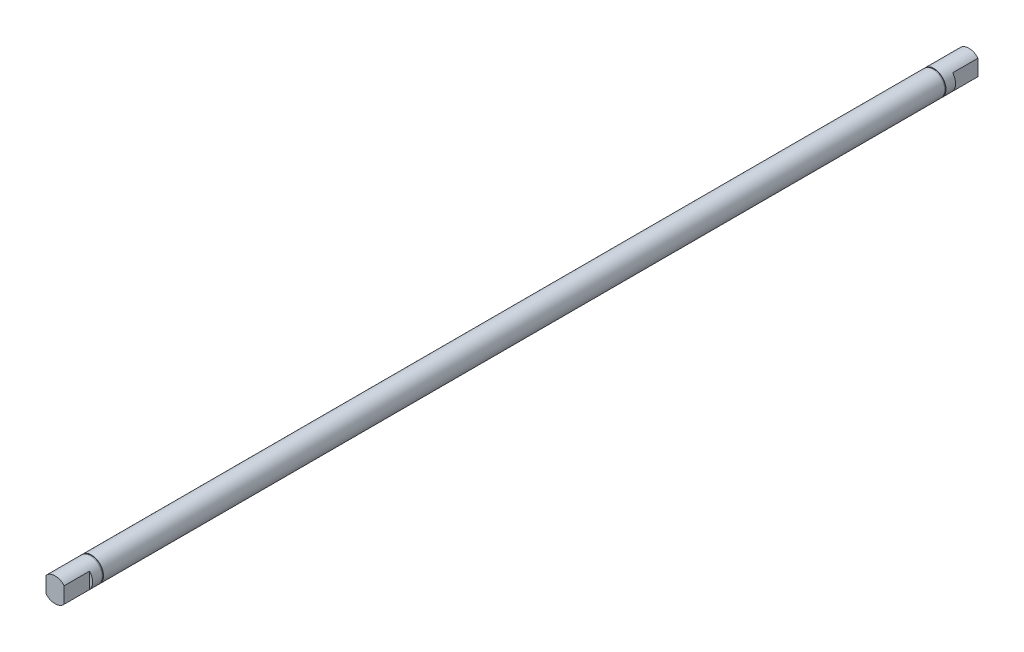
from build123d import *

# Parameters (mm, degrees)
SKETCH_1_R          = 10
EXTRUDE_1_DEPTH     = 377.5
SKETCH_2_W          = 20.903935991
SKETCH_2_H          = 21
CUT_EXTRUDE_1_DEPTH = 25
CUT_EXTRUDE_START   = -30
SKETCH_5_R          = 10
SKETCH_5_R_2        = 9.5
CUT_EXTRUDE_2_DEPTH = 1.1


with BuildPart() as part:
    # 草图1 → 凸台-拉伸1 (new, symmetric)
    with BuildSketch(Plane.XY):
        Circle(SKETCH_1_R)
    extrude(amount=EXTRUDE_1_DEPTH, both=True)

    # 草图2 → 切除-拉伸1 (cut, symmetric)
    with BuildSketch(Plane(origin=(0, 0, 0), x_dir=(1, 0, 0), z_dir=(0, 1, 0))):
        with Locations((-17.951967996, 367)):
            Rectangle(SKETCH_2_W, SKETCH_2_H)
        with Locations((17.951967996, 367)):
            Rectangle(SKETCH_2_W, SKETCH_2_H)
        with Locations((17.951967996, -367)):
            Rectangle(SKETCH_2_W, SKETCH_2_H)
        with Locations((-17.951967996, -367)):
            Rectangle(SKETCH_2_W, SKETCH_2_H)
    extrude(amount=CUT_EXTRUDE_1_DEPTH, both=True, mode=Mode.SUBTRACT)

    # 草图5 → 切除-拉伸2 (cut)
    with BuildSketch(Plane(origin=(0, 0, -377.5), x_dir=(-1, 0, 0), z_dir=(0, 0, -1)).offset(CUT_EXTRUDE_START)):
        Circle(SKETCH_5_R)
        Circle(SKETCH_5_R_2, mode=Mode.SUBTRACT)
    cut_extrude_2 = extrude(amount=CUT_EXTRUDE_2_DEPTH, mode=Mode.SUBTRACT)

    # 镜向1: 切除-拉伸2 across plane
    add(cut_extrude_2.mirror(Plane.XY), mode=Mode.SUBTRACT)


solid = part.part
